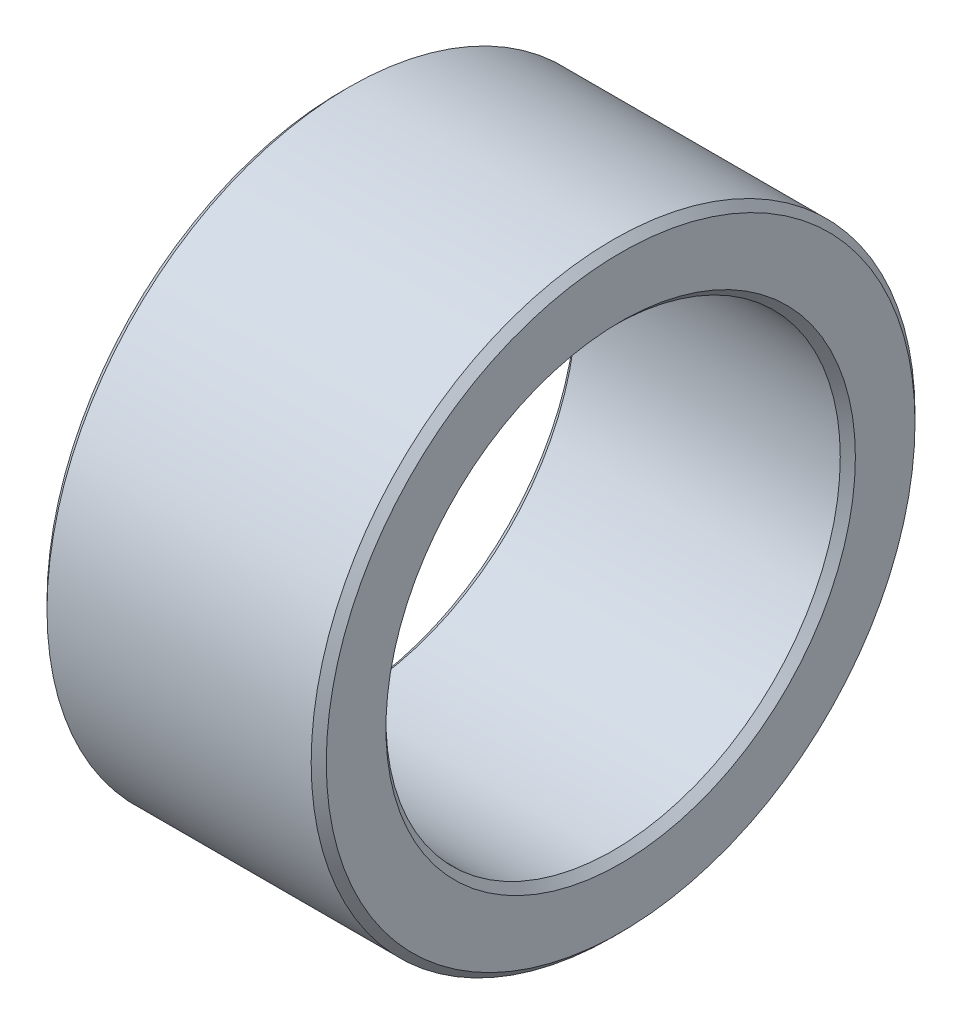
SolidWorks part; units mm, degrees
material "45#"
ref_plane "前基準面" through (0, 0, 0) normal (0, 0, 1) x (1, 0, 0)
ref_plane "上基準面" through (0, 0, 0) normal (0, 1, 0) x (1, 0, 0)
ref_plane "右基準面" through (0, 0, 0) normal (1, 0, 0) x (0, 0, -1)
sketch "草图1" plane through (0, 0, 0) normal (1, 0, 0) x (0, 0, -1)
  circle A0 centre (0, 0) radius 15.05
  circle A1 centre (0, 0) radius 20
  dimension "D1" = 30.1
  dimension "D2" = 40
extrude "凸台-拉伸1" add sketch "草图1" along normal blind 18.5
chamfer "倒角1" distance 0.5 angle 45 4 edges at (0, 0, -15.05) (18.5, 0, -15.05) (0, 0, -20) (18.5, 0, -20)
